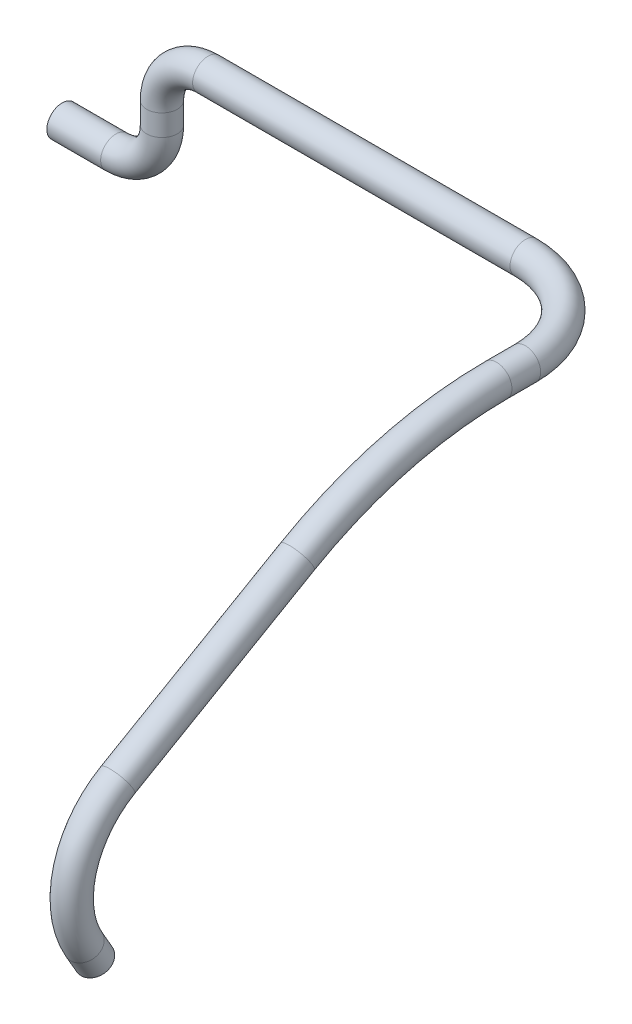
SolidWorks part; units mm, degrees
ref_plane "Front Plane" through (0, 0, 0) normal (0, 0, 1) x (1, 0, 0)
ref_plane "Top Plane" through (0, 0, 0) normal (0, 1, 0) x (1, 0, 0)
ref_plane "Right Plane" through (0, 0, 0) normal (1, 0, 0) x (0, 0, -1)
sketch3d "3DSketch1"
  line L0 (-50.1983, 33.7799, 68.3045) -> (-50.1909, 36.1641, 69.6806)
  line L1 (-50.1983, 33.7799, 68.3045) -> (-50.1983, 36.7669, 63.129) construction
  line L2 (-50.1589, 52.5557, 65.2857) -> (-50.1589, 66.0808, 41.8515)
  line L4 (-122.5983, 58.2636, 0.1096) -> (-115.5778, 58.2636, 0.1096)
  line L5 (-109.5778, 64.2636, 0.1096) -> (-109.5778, 67.0436, 0.1096)
  line L6 (-103.5778, 73.0436, 0.1096) -> (-62.1589, 73.0436, 0.1096)
  line L7 (-50.1589, 73.0436, 15.8583) -> (-50.1589, 73.0436, 12.1096)
  arc A2 (-50.1589, 73.0436, 15.8583) -> (-50.1589, 66.0808, 41.8515) centre (-50.1589, 21.0436, 15.8583) ccw
  arc A3 (-50.1909, 36.1641, 69.6806) -> (-50.1589, 52.5557, 65.2857) centre (-50.1909, 42.1626, 59.2873) ccw
  arc A4 (-62.1589, 73.0436, 0.1096) -> (-50.1589, 73.0436, 12.1096) centre (-62.1589, 73.0436, 12.1096) ccw
  arc A5 (-103.5778, 73.0436, 0.1096) -> (-109.5778, 67.0436, 0.1096) centre (-103.5778, 67.0436, 0.1096) ccw
  arc A6 (-109.5778, 64.2636, 0.1096) -> (-115.5778, 58.2636, 0.1096) centre (-115.5778, 64.2636, 0.1096) ccw
  point P18 (-50.1589, 73.0436, 29.7874)
  point P19 (1.8411, 21.0436, 15.8583)
  point P22 (-50.1589, 46.5573, 75.679)
  point P23 (-62.1909, 42.1903, 59.3033)
  point P26 (-50.1589, 73.0436, 0.1096)
  point P27 (-62.1589, 61.0436, 12.1096)
  point P30 (-109.5778, 73.0436, 0.1096)
  point P31 (-103.5778, 67.0436, 6.1096)
  point P34 (-109.5778, 58.2636, 0.1096)
  point P35 (-115.5778, 64.2636, -5.8904)
  dimension "D1" = 52
  dimension "D2" = 12
  dimension "D3" = 12
  dimension "D4" = 6
ref_plane "Plane1" through (-122.5983, 0, 0) normal (1, 0, 0) x (0, 0, -1)
sketch "Sketch1" plane through (-122.5983, 0, 0) normal (1, 0, 0) x (0, 0, -1)
  circle A0 centre (-0.1096, 58.2636) radius 2
  dimension "D1" = 4
sweep "Sweep1" add profiles "Sketch1" path "3DSketch1"
